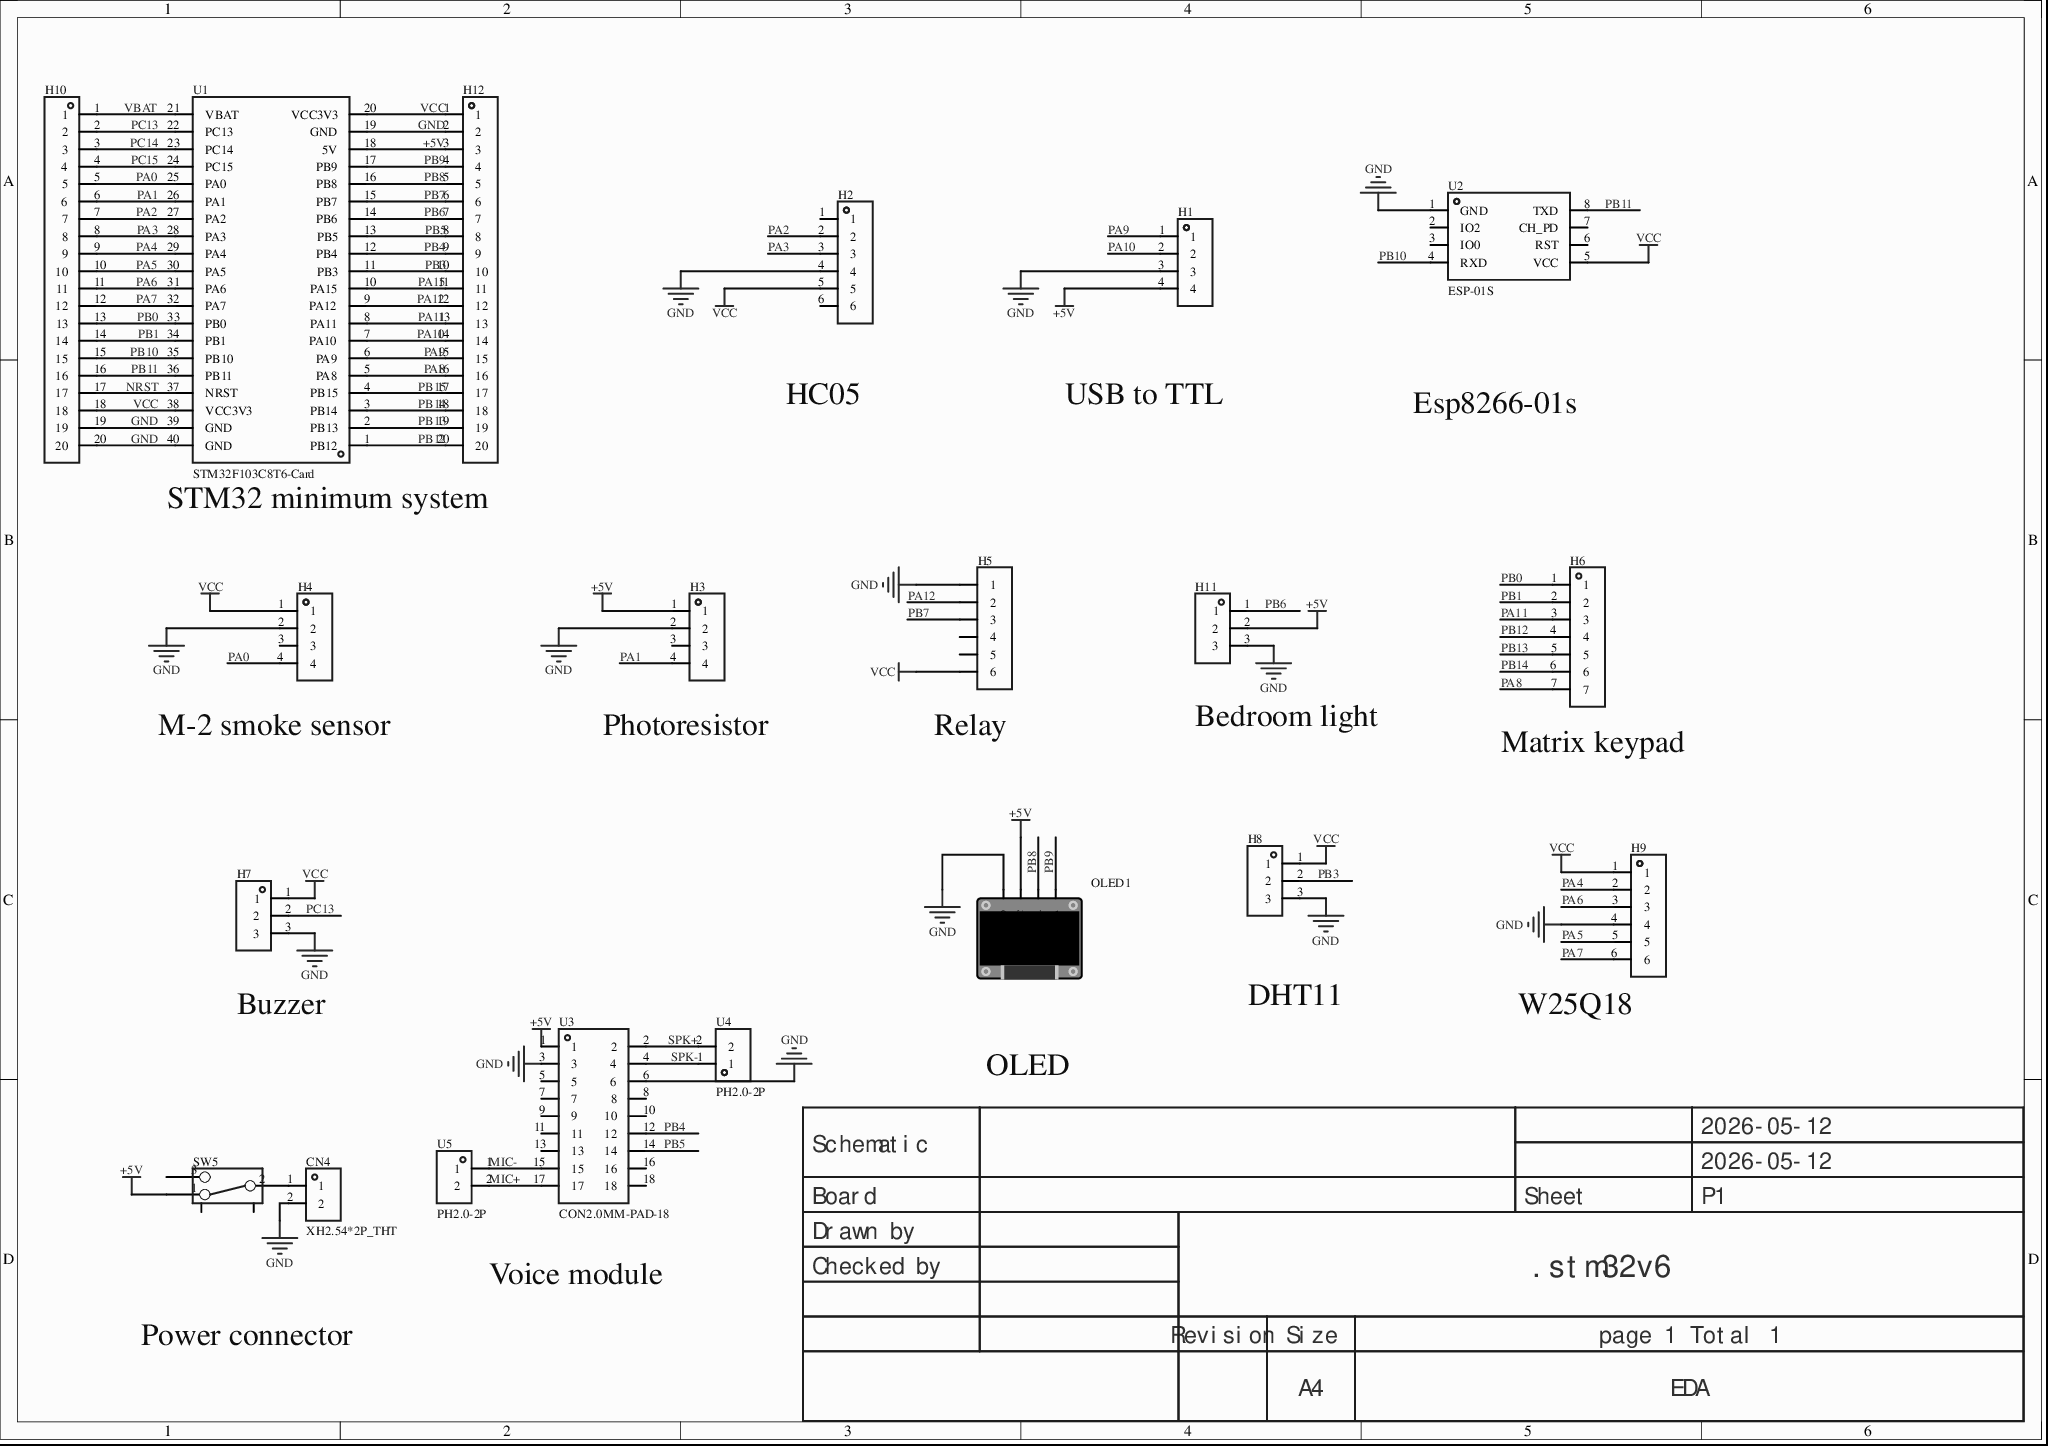
[diagram p0: MISC49851-3.schdoc]
# Altium project MISC49851-2.PrjPcb
1 sheet, 20 parts. Net scope: global (net labels, ports and power ports of the same name join across sheets).
Board file: MISC49851.pcbdoc

## Sheet MISC49851-3.schdoc
size 297 x 209 mm; Version: V1.0; @Project Name: MISC49851; @Page Count: 1; @Update Date: 2026-05-12; @Create Date: 2026-05-12; @Schematic Name: MISC49851; @Page No: 1; @Create Time: 23:22:16; @Update Time: 17:32:40; @Board Name: MISC49851

### Parts
CN4  XH2.54*2P_THT  [CONN-TH_2P-P2.50-XH2.54-2P]
H1  (no value)  [HDR-TH_4P-P2.54-V-F]
H2  (no value)  [HDR-TH_6P-P2.54-V-F]
H3  (no value)  [HDR-TH_4P-P2.54-V-F]
H4  (no value)  [HDR-TH_4P-P2.54-V-F]
H5  (no value)  [HDR-TH_6P-P2.54-V-M-1]
H6  (no value)  [HDR-TH_7P-P2.54-V-M]
H7  (no value)  [HDR-TH_3P-P2.54-V-F]
H8  (no value)  [HDR-TH_3P-P2.54-V-F]
H9  (no value)  [HDR-TH_6P-P2.54-V-F]
H10  (no value)  [HDR-TH_20P-P2.54-V-M-1]
H11  (no value)  [HDR-TH_3P-P2.54-V-F]
H12  (no value)  [HDR-TH_20P-P2.54-V-M-1]
OLED1  (no value)  [0.96OLED_4P]
SW5  (no value)  [拨动开关]
U1  STM32F103C8T6-Card  [CONN-TH_L53.3-W22.9_STM32F103C8T6-CARD]
U2  ESP-01S  [WIFIM-TH_ESP-01S]
U3  CON2.0MM-PAD-18  [CONN-TH_18P-P2.00_C9900078766]
U4  PH2.0-2P  [CONN-TH_2P-P2.00_BOSSIE_BX-PH2.0-2PZZ]
U5  PH2.0-2P  [CONN-TH_2P-P2.00_BOSSIE_BX-PH2.0-2PZZ]

### Nets
+5V: H1.4 H3.1 H11.2 H12.3 OLED1.2(VCC) SW5.1 U1.18(5V) U3.1
GND: CN4.2 H1.3 H2.4 H3.2 H4.2 H5.1 H7.3 H8.3 H9.4 H10.19 H10.20 H11.3 H12.2 OLED1.1(GND) U1.19(GND) U1.39(GND) U1.40(GND) U2.1(GND) U3.3 U3.6
VCC: H2.5 H4.1 H5.6 H7.1 H8.1 H9.1 H10.18 H12.1 U1.20(VCC3V3) U1.38(VCC3V3) U2.5(VCC)
MIC+: U3.17 U5.2
MIC-: U3.15 U5.1
NRST: H10.17 U1.37(NRST)
PA0: H4.4 H10.5 U1.25(PA0)
PA1: H3.4 H10.6 U1.26(PA1)
PA2: H2.2 H10.7 U1.27(PA2)
PA3: H2.3 H10.8 U1.28(PA3)
PA4: H9.2 H10.9 U1.29(PA4)
PA5: H9.5 H10.10 U1.30(PA5)
PA6: H9.3 H10.11 U1.31(PA6)
PA7: H9.6 H10.12 U1.32(PA7)
PA8: H6.7 H12.16 U1.5(PA8)
PA9: H1.1 H12.15 U1.6(PA9)
PA10: H1.2 H12.14 U1.7(PA10)
PA11: H6.3 H12.13 U1.8(PA11)
PA12: H5.2 H12.12 U1.9(PA12)
PA15: H12.11 U1.10(PA15)
PB0: H6.1 H10.13 U1.33(PB0)
PB1: H6.2 H10.14 U1.34(PB1)
PB3: H8.2 H12.10 U1.11(PB3)
PB4: H12.9 U1.12(PB4) U3.12
PB5: H12.8 U1.13(PB5) U3.14
PB6: H11.1 H12.7 U1.14(PB6)
PB7: H5.3 H12.6 U1.15(PB7)
PB8: H12.5 OLED1.3(SCL) U1.16(PB8)
PB9: H12.4 OLED1.4(SDA) U1.17(PB9)
PB10: H10.15 U1.35(PB10) U2.4(RXD)
PB11: H10.16 U1.36(PB11) U2.8(TXD)
PB12: H6.4 H12.20 U1.1(PB12)
PB13: H6.5 H12.19 U1.2(PB13)
PB14: H6.6 H12.18 U1.3(PB14)
PB15: H12.17 U1.4(PB15)
PC13: H7.2 H10.2 U1.22(PC13)
PC14: H10.3 U1.23(PC14)
PC15: H10.4 U1.24(PC15)
SPK+: U3.2 U4.2
SPK-: U3.4 U4.1
VBAT: H10.1 U1.21(VBAT)
NetCN4_1: CN4.1 SW5.2

Not connected (* = marked no-connect by the designer): H2 1 6; H3 3; H4 3; H5 4 5; SW5 3 4 5; U2 2(IO2)* 3(IO0)* 6(RST)* 7(CH_PD)*; U3 5 7 8 9 10 11 13 16 18

### Notes on the sheet
- 串口：
  蓝牙               PA2,PA3
  USB转TTL  		PA10，PA9
  ESP8266-01s        PB10,PB11
  GPIO:
  MQ-2 烟雾报警器  PA0
  光敏电阻 PA1
  卧室灯 PA11   5V
  矩阵键盘  PA8,PB0,PB1,PB2,PB12,PB13,PB14
  SU-03T  PB4,PB5
  蜂鸣器 PC13
  IIC:
  0.96英寸OLED显示屏	PB8，PB9
  One-Wire:
  DHT11  PB3
  SPI:
  W25Q128 PA4,PA5,PA6,PA7   3v3
- HC05
- USB to TTL
- Esp8266-01s
- STM32 minimum system
- (near H4) M-2 smoke sensor
- (near H3) Photoresistor
- (near H5) Relay
- (near H11) Bedroom light
- (near H6) Matrix keypad
- (near H7) Buzzer
- DHT11
- (near H9) W25Q18
- OLED
- Voice module
- Power connector
- Labels drawn without touching a wire or pin: VCC
- 2026-05-12
- Schematic
- Board
- Sheet
- P1
- Drawn by
- Checked by
- .stm32v6
- Revision
- Size
- A4
- page 1 Total 1
- EDA

### Library data of the parts
CN4 = XH2.54*2P_直插: 3D Model: 325c595e30db4df8abe76612dd40b0fa0819f05c4eef4c71ace90d822a990e87; 3D Model Transform: 295.275,228.346,0,180,0,0,-0.002,-20.079,-137.795; AddInBom: yes; Symbol: XH2.54*2P_THT; Device: XH2.54*2P_THT; LCSC Part Name: XH2.54*2P_直插; Supplier Part: C9900008615; Manufacturer Part: XH2.54*2P_直插; Supplier Footprint: XH2.54_2P; JLCPCB Part Class: Extended Part; Supplier: LCSC; ConvertToPcb: yes; FootprintName: CONN-TH_2P-P2.50-XH2.54-2P; ModelName: CONN-TH_2P-P2.50-XH2.54-2P
H1 H3 H4 = HDR-F_2.54_1x4P: Symbol: 2.54-1*4P female; 3D Model: d187812051054f85879fcaa51a310d8e0819f05c4eef4c71ace90d822a990e87; 3D Model Transform: 419.6842,98.464,0,0,0,0,0,0,-118.11; ConvertToPcb: yes; Device: HDR-F_2.54_1x4P; Supplier Part: C2718488; Supplier Footprint: 插件; FootprintName: HDR-TH_4P-P2.54-V-F; AddInBom: yes; ModelName: HDR-TH_4P-P2.54-V-F
H2 H9 = HDR-F_2.54_1x6P: Symbol: Header-Female-2.54_1x6; ConvertToPcb: yes; ModelId: 0f5bcf94dcda47d085f24cdca1696fe9; ModelTransform: 619.684,94.488,0,0,0,0,0,0,-125.984; Device: HDR-F_2.54_1x6P; AddInBom: yes; SupplierPart: C40877; Supplier Footprint: 插件; FootprintName: HDR-TH_6P-P2.54-V-F; ModelName: HDR-TH_6P-P2.54-V-F
H5 = HDR-M_2.54_1x6P: Symbol: Header-Male-2.54_1x6; ConvertToPcb: yes; ModelId: 60739dffc9b04830a286435b0fefbd4a0819f05c4eef4c71ace90d822a990e87; ModelName: HDR2.54-M-LI-1X6P; ModelTransform: 599.999,100,0,0,0,0,0,0,-118.11; Device: HDR-M_2.54_1x6P; AddInBom: yes; SupplierPart: C37208; Supplier Footprint: 插件; FootprintName: HDR-TH_6P-P2.54-V-M-1
H6 = HDR-M_2.54_1x7P: Symbol: PZ254V-11-07P; ConvertToPcb: yes; ModelId: 3f496cdc752348c6a5e9157bbaceaf960819f05c4eef4c71ace90d822a990e87; ModelName: HDR-TH_7P-P2.54-M-LI-1X7P; ModelTransform: 690.1561,98.425,0,0,0,0,0,0,-118.11; Device: HDR-M_2.54_1x7P; AddInBom: yes; SupplierPart: C492406; Supplier Footprint: 插件; FootprintName: HDR-TH_7P-P2.54-V-M
H7 H8 H11 = HDR-F_2.54_1x3P: Symbol: PM254V-11-03-H85; 3D Model: f3b3cc5aae9641bf9e56fc160cef875b; 3D Model Transform: 299.9994,100,0,0,0,0,0,0,-118.11; ConvertToPcb: yes; ModelName: HDR2.54-F-LI-1X3P; Device: HDR-F_2.54_1x3P; Supplier Part: C541850; Supplier Footprint: 插件; AddInBom: yes; FootprintName: HDR-TH_3P-P2.54-V-F
H10 H12 = HDR-M_2.54_1x20P: 间距:2.54mm;总PIN位数:20;排数:1;插针结构:-;行距:-;安装类型:直插;圆针/方针:-;额定电流:-;额定电压:-;配合针长度:-;塑高:-;触头材质:黄铜;触头镀层:-;颜色:黑色;; Symbol: HDR_2.54-1x20P; ConvertToPcb: yes; ModelId: f68709be121d406db68b06f32a5953890819f05c4eef4c71ace90d822a990e87; ModelName: HDR-M-2.54_1x20; ModelTransform: 1999.996,100,0,0,0,0,0,0,-118.11; Device: HDR-M_2.54_1x20P; AddInBom: yes; SupplierPart: C50981; Supplier Footprint: 插件; FootprintName: HDR-TH_20P-P2.54-V-M-1
OLED1 = 0.96OLED模块_4P: Symbol: 0.96OLED module_4P; ConvertToPcb: yes; ModelId: 79c000fdb68d45a296c2e9bedf4f9055; ModelTransform: 1393.69792,1318.895,0,0,0,0,0,-560.079,-137.795; Device: 0.96OLED module_4P; AddInBom: yes; FootprintName: 0.96OLED_4P; Supplier Footprint: 插件; ModelName: 0.96OLED_4P
SW5 = 拨动开关_正: Symbol: Toggle switch; Device: Toggle switch_positive; ConvertToPcb: yes; ModelId: 4321fe59a4074cbfb4989553f297c68f0819f05c4eef4c71ace90d822a990e87; ModelName: SW-TH_SS-12D02-VG4; ModelTransform: 370.09,208.7,472.35,0,0,0,0,0,-110; AddInBom: yes; Supplier Footprint: 插件; FootprintName: Toggle switch
U1 = STM32F103C8T6-Card: AddInBom: yes; Symbol: STM32F103C8T6-CARD; Device: STM32F103C8T6-Card; LCSC Part Name: STM32F103C8T6-Card; SupplierPart: C9900077949; ManufacturerPart: STM32F103C8T6-Card; Supplier Footprint: 插件; Supplier: LCSC; ConvertToPcb: yes; FootprintName: CONN-TH_L53.3-W22.9_STM32F103C8T6-CARD
U2 = ESP-01S_C111009: AddInBom: yes; ModelId: eb7175da78ae48b3b1568cfe3027405f0819f05c4eef4c71ace90d822a990e87; ModelTransform: 582.676,976.37608,0,0,0,0,0,388.346,-118.11; Symbol: ESP-01S; Device: ESP-01S_C111009; LCSC Part Name: ESP-01S; SupplierPart: C111009; ManufacturerPart: ESP-01S; Supplier Footprint: -; JLCPCB Part Class: Extended Part; Supplier: LCSC; ConvertToPcb: yes; FootprintName: WIFIM-TH_ESP-01S; ModelName: WIFIM-TH_ESP-01S
U3 = CON2.0MM-PAD-18: AddInBom: yes; ModelId: 07100c6dd3a4442ea12d6f5a4e41c4c80819f05c4eef4c71ace90d822a990e87; ModelTransform: 787.7937,374.015,0,0,0,0,0,-14.961,-118.11; Symbol: CON2.0MM-PAD-18; Device: CON2.0MM-PAD-18; LCSC Part Name: CON2.0MM-PAD-18; SupplierPart: C9900078766; ManufacturerPart: CON2.0MM-PAD-18; Supplier Footprint: TH-2*9P-2.0; JLCPCB Part Class: Extended Part; Supplier: LCSC; ConvertToPcb: yes; FootprintName: CONN-TH_18P-P2.00_C9900078766; ModelName: CONN-TH_18P-P2.00_C9900078766
U4 = PH2.0-2P: Symbol: PH2.0-2P_C9900095162; 3D Model: d36e580ea2964da0aea981f13f36722f0819f05c4eef4c71ace90d822a990e87; 3D Model Transform: 236.22,185.4327,0,0,0,0,-0.591,-22.244,-137.795; AddInBom: yes; Device: PH2.0-2P; LCSC Part Name: PH2.0-2P; Supplier Part: C9900095162; Manufacturer Part: PH2.0-2P; Supplier Footprint: CONN-TH_2P-P2.00_BOSSIE_BX-PH2.0-2PZZ; JLCPCB Part Class: Extended Part; Supplier: LCSC; ConvertToPcb: yes; FootprintName: CONN-TH_2P-P2.00_BOSSIE_BX-PH2.0-2PZZ; ModelName: CONN-TH_2P-P2.00_BOSSIE_BX-PH2.0-2PZZ
U5 = PH2.0-2P: Symbol: PH2.0-2P_C9900095162; AddInBom: yes; ModelId: d36e580ea2964da0aea981f13f36722f0819f05c4eef4c71ace90d822a990e87; ModelTransform: 236.22,185.4327,0,0,0,0,-0.591,-22.244,-137.795; Device: PH2.0-2P; LCSC Part Name: PH2.0-2P; SupplierPart: C9900095162; ManufacturerPart: PH2.0-2P; Supplier Footprint: CONN-TH_2P-P2.00_BOSSIE_BX-PH2.0-2PZZ; JLCPCB Part Class: Extended Part; Supplier: LCSC; ConvertToPcb: yes; FootprintName: CONN-TH_2P-P2.00_BOSSIE_BX-PH2.0-2PZZ; ModelName: CONN-TH_2P-P2.00_BOSSIE_BX-PH2.0-2PZZ